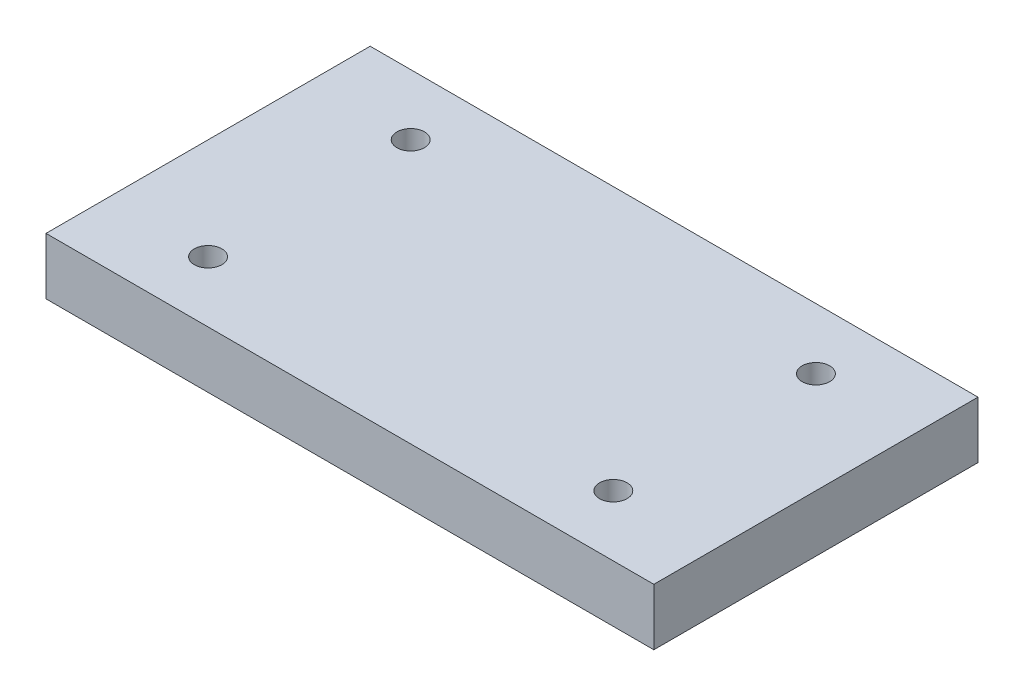
SolidWorks part; units mm, degrees
material "普通碳钢"
ref_plane "Front Plane" through (0, 0, 0) normal (0, 0, 1) x (1, 0, 0)
ref_plane "Top Plane" through (0, 0, 0) normal (0, 1, 0) x (1, 0, 0)
ref_plane "Right Plane" through (0, 0, 0) normal (1, 0, 0) x (0, 0, -1)
sketch "Sketch1" plane through (0, 0, 0) normal (0, 1, 0) x (1, 0, 0)
  line L1 (0, 0) -> (150, 0)
  line L2 (0, 0) -> (0, 80)
  line L3 (0, 80) -> (150, 80)
  line L4 (150, 0) -> (150, 80)
  dimension "D1" = 80
  dimension "D2" = 150
extrude "Boss-Extrude1" add sketch "Sketch1" along normal blind 14
hole_wizard "M8 Tapped Hole1" positions "Sketch2" profile "Sketch3" tap size "M8" standard "GB" end condition through all
sketch "Sketch2" plane through (0, 14, 0) normal (0, 1, 0) x (-1, 0, 0)
  line L0 (-25, -65) -> (-125, -65) construction
  line L1 (-125, -65) -> (-125, -15) construction
  line L2 (-125, -15) -> (-25, -15) construction
  line L3 (-25, -15) -> (-25, -65) construction
  line L5 (-75, -65) -> (-75, -80) construction
  line L6 (-150, -80) -> (0, -80) construction
  line L8 (-25, -40) -> (0, -40) construction
  line L9 (0, -80) -> (0, 0) construction
  point P0 (-25, -65)
  point P2 (-25, -15)
  point P4 (-125, -15)
  point P6 (-125, -65)
  dimension "D1" = 50
  dimension "D2" = 100
sketch "Sketch3" plane through (25, 14, -65) normal (1, 0, 0) x (0, 0, 1)
  line L0 (0, 0) -> (0, 14)
  line L1 (0, 14) -> (3.4, 14)
  line L2 (3.4, 14) -> (3.4, 0)
  line L5 (3.4, 0) -> (0, 0)
  line L11 (0, -6.35) -> (0, 107.95) construction
  dimension "通孔螺纹孔钻头直径" = 6.8
  dimension "通孔螺纹孔钻头深度" = 14
cosmetic thread "Hole cosmetic thread1"
cosmetic thread "Hole cosmetic thread2"
cosmetic thread "Hole cosmetic thread3"
cosmetic thread "Hole cosmetic thread4"
